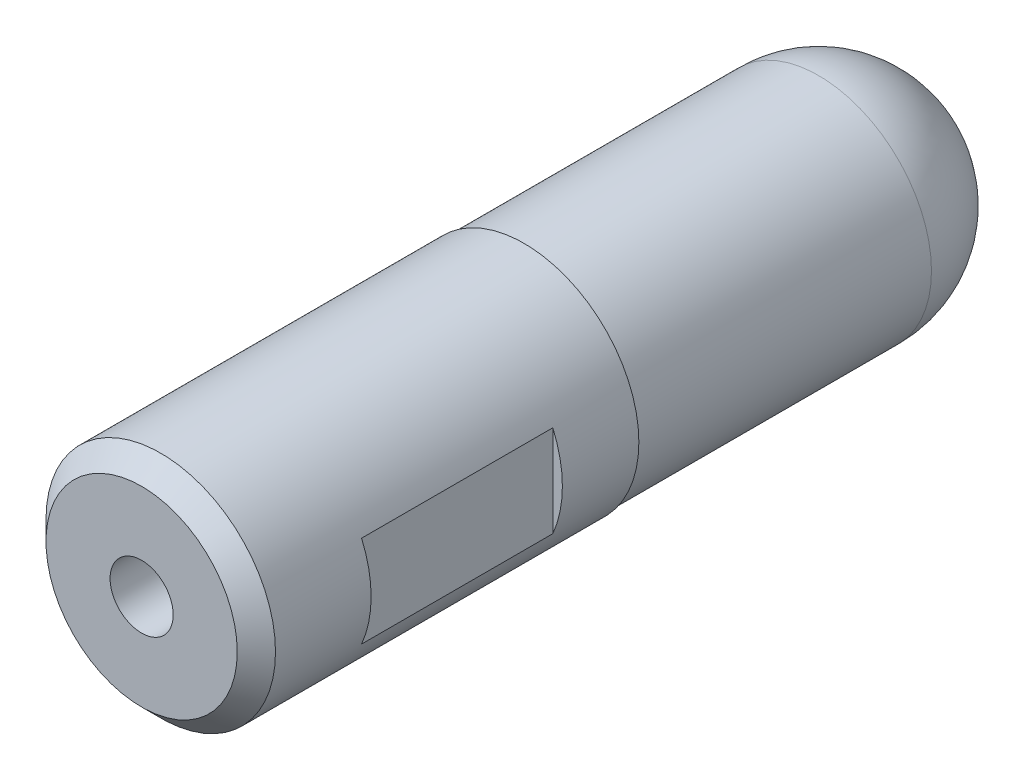
SolidWorks part; units mm, degrees
material "AISI 304"
ref_plane "Front Plane" through (0, 0, 0) normal (0, 0, 1) x (1, 0, 0)
ref_plane "Top Plane" through (0, 0, 0) normal (0, 1, 0) x (1, 0, 0)
ref_plane "Right Plane" through (0, 0, 0) normal (1, 0, 0) x (0, 0, -1)
sketch "Sketch1" plane through (0, 0, 0) normal (0, 0, 1) x (1, 0, 0)
  circle A0 centre (0, 0) radius 5.9
  dimension "D1" = 11.8
extrude "Boss-Extrude1" add sketch "Sketch1" along normal blind 35.4
sketch "Sketch2" plane through (0, 0, 0) normal (0, 1, 0) x (1, 0, 0)
  line L0 (0, 5.9) -> (0, 0)
  line L1 (0, 0) -> (-5.9, 0)
  arc A0 (0, 5.9) -> (-5.9, 0) centre (0, 0) ccw
  dimension "D1" = 11.8
revolve "Revolve1" add sketch "Sketch2" angle 360 about L0
hole_wizard "M4 Tapped Hole1" positions "Sketch3" profile "Sketch4" tap size "M4" standard "GB"
sketch "Sketch3" plane through (0, 0, 35.4) normal (0, 0, 1) x (1, 0, 0)
  point P0 (0, 0)
sketch "Sketch4" plane through (0, 0, 35.4) normal (1, 0, 0) x (0, -1, 0)
  line L0 (0, 0) -> (0, 11.0914)
  line L1 (0, 11.0914) -> (1.65, 10.1)
  line L2 (1.65, 10.1) -> (1.65, 0)
  line L5 (1.65, 0) -> (0, 0)
  line L10 (0, 11.0914) -> (-1.65, 10.1) construction
  line L11 (0, -6.35) -> (0, 107.95) construction
  dimension "螺纹孔钻头直径" = 3.3
  dimension "螺纹孔钻头深度" = 10.1
  dimension "导头角度" = 118
cosmetic thread "Cosmetic thread 1"
sketch "Sketch5" plane through (0, 0, 35.4) normal (0, 0, 1) x (1, 0, 0)
  circle A0 centre (0, 0) radius 6
  circle A1 centre (0, 0) radius 4
  dimension "D1" = 12
  dimension "D2" = 8
extrude "Boss-Extrude2" add sketch "Sketch5" against normal blind 20
chamfer "Chamfer1" distance 1 angle 45 1 edges at (6, 0, 35.4)
sketch "Sketch6" plane through (0, 0, 0) normal (0, 1, 0) x (1, 0, 0)
  line L0 (-5, -35.4) -> (5, -35.4) construction
  line L1 (-7.5263, -19.4) -> (-5.5, -19.4)
  line L2 (-7.5263, -19.4) -> (-7.5263, -29.4)
  line L3 (-7.5263, -29.4) -> (-5.5, -29.4)
  line L4 (-5.5, -19.4) -> (-5.5, -29.4)
  line L5 (7.5263, -19.4) -> (5.5, -19.4)
  line L6 (7.5263, -19.4) -> (7.5263, -29.4)
  line L7 (7.5263, -29.4) -> (5.5, -29.4)
  line L8 (5.5, -19.4) -> (5.5, -29.4)
  line L9 (0, -35.4) -> (0, -40.7235) construction
  dimension "D1" = 11
  dimension "D2" = 6
  dimension "D3" = 10
extrude "Cut-Extrude1" cut sketch "Sketch6" against normal through all both and the other way through all
